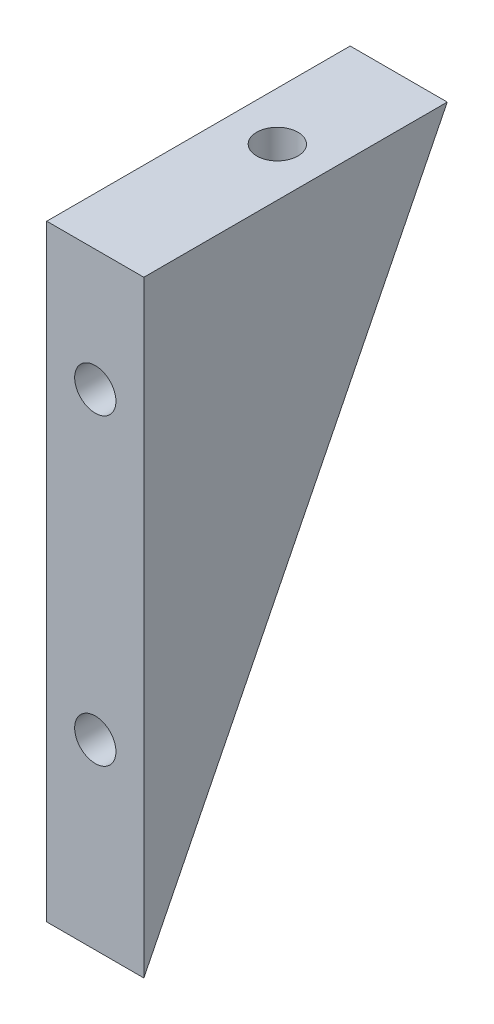
from build123d import *

# Parameters (mm, degrees)
EXTRUDE_1_DEPTH        = 16
HOLE_WIZARD_M8_1_D     = 6.8
HOLE_WIZARD_M8_1_DEPTH = 29.25
HOLE_WIZARD_M8_1_TIP   = 2.042926105
HOLE_WIZARD_M8_2_D     = 6.8
HOLE_WIZARD_M8_2_DEPTH = 29.25
HOLE_WIZARD_M8_2_TIP   = 2.042926105


with BuildPart() as part:
    # 草图1 → 凸台-拉伸1 (new body)
    with BuildSketch(Plane(origin=(0, 0, 0), x_dir=(0, 0, -1), z_dir=(1, 0, 0))):
        Polygon((0, 0), (50, 0), (0, -100), align=None)
    extrude(amount=EXTRUDE_1_DEPTH)

    # M8 螺纹孔1
    with Locations(Plane(origin=(0, 0, 0), x_dir=(1, 0, 0), z_dir=(0, 1, 0))):
        with Locations((8, 30)):
            Hole(HOLE_WIZARD_M8_1_D / 2, depth=HOLE_WIZARD_M8_1_DEPTH)
            with Locations((0, 0, -(HOLE_WIZARD_M8_1_DEPTH + HOLE_WIZARD_M8_1_TIP / 2))):  # 118° drill point
                Cone(0, HOLE_WIZARD_M8_1_D / 2, HOLE_WIZARD_M8_1_TIP, mode=Mode.SUBTRACT)

    # M8 螺纹孔2
    with Locations(Plane.XY):
        with Locations((8, -20), (8, -70)):
            Hole(HOLE_WIZARD_M8_2_D / 2, depth=HOLE_WIZARD_M8_2_DEPTH)
            with Locations((0, 0, -(HOLE_WIZARD_M8_2_DEPTH + HOLE_WIZARD_M8_2_TIP / 2))):  # 118° drill point
                Cone(0, HOLE_WIZARD_M8_2_D / 2, HOLE_WIZARD_M8_2_TIP, mode=Mode.SUBTRACT)


solid = part.part
